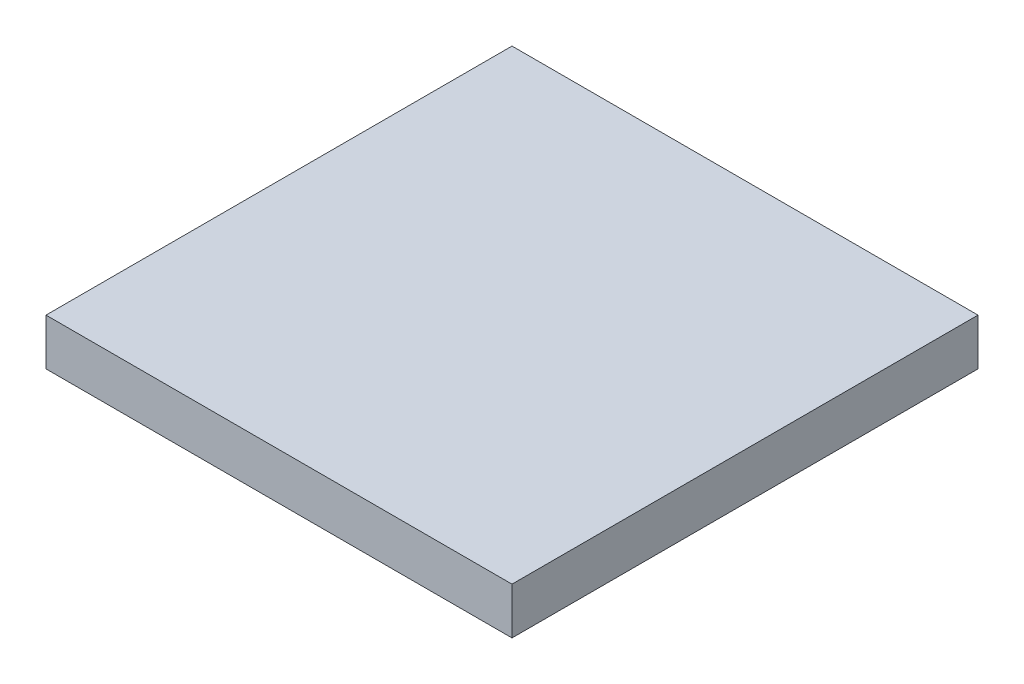
SolidWorks part; units mm, degrees
ref_plane "前视基准面" through (0, 0, 0) normal (0, 0, 1) x (1, 0, 0)
ref_plane "上视基准面" through (0, 0, 0) normal (0, 1, 0) x (1, 0, 0)
ref_plane "右视基准面" through (0, 0, 0) normal (1, 0, 0) x (0, 0, -1)
sketch "草图1" plane through (0, 0, 0) normal (0, 1, 0) x (1, 0, 0)
  line L1 (-250, 250) -> (250, 250)
  line L2 (-250, 250) -> (-250, -250)
  line L3 (-250, -250) -> (250, -250)
  line L4 (250, 250) -> (250, -250)
  line L5 (-250, 250) -> (250, -250) construction
  line L6 (-250, -250) -> (250, 250) construction
  point P0 (0, 0)
  dimension "D1" = 500
  dimension "D2" = 500
extrude "凸台-拉伸1" add sketch "草图1" along normal blind 50
